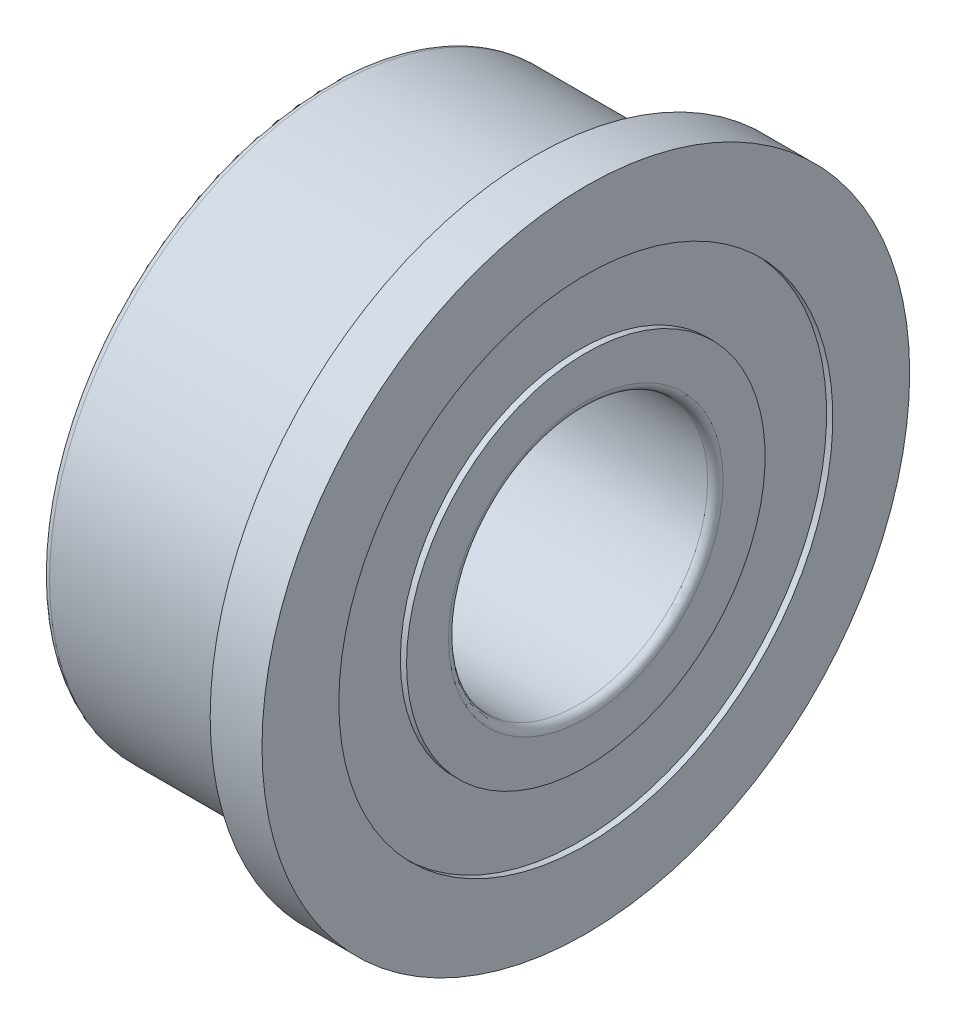
from build123d import *


with BuildPart() as part:
    # Sketch1 → Revolve1 (revolve)
    with BuildSketch(Plane.XY, mode=Mode.PRIVATE) as revolve1_sk:
        with BuildLine():
            Line((0, 5.35), (0, 4.767))
            Line((0, 4.767), (0.12, 4.767))
            Line((0.12, 4.767), (0.12, 3.46))
            Line((0.12, 3.46), (0, 3.46))
            Line((0, 3.46), (0, 2.65))
            ThreePointArc((0, 2.65), (0.043933983, 2.543933983), (0.15, 2.5))
            Line((0.15, 2.5), (4.85, 2.5))
            ThreePointArc((4.85, 2.5), (4.956066017, 2.543933983), (5, 2.65))
            Line((5, 2.65), (5, 3.46))
            Line((5, 3.46), (4.88, 3.46))
            Line((4.88, 3.46), (4.88, 4.767))
            Line((4.88, 4.767), (5, 4.767))
            Line((5, 4.767), (5, 6.25))
            Line((5, 6.25), (4, 6.25))
            Line((4, 6.25), (4, 5.65))
            ThreePointArc((4, 5.65), (4.106066017, 5.393933983), (3.85, 5.5))
            Line((3.85, 5.5), (0.15, 5.5))
            ThreePointArc((0.15, 5.5), (0.043933983, 5.456066017), (0, 5.35))
        make_face()
    revolve(revolve1_sk.sketch.rotate(Axis((11, 0, 0), (-1, 0, 0)), 270), axis=Axis((11, 0, 0), (-1, 0, 0)))


solid = part.part
